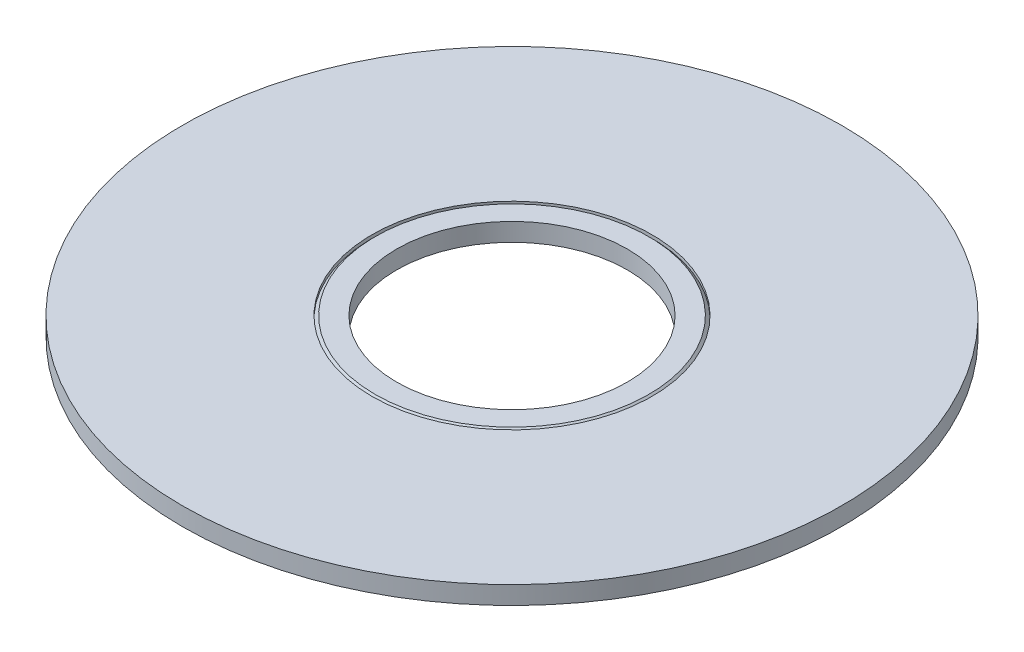
from build123d import *

# Parameters (mm, degrees)
SKETCH1_R           = 42.5
SKETCH1_R_2         = 35
BOSS_EXTRUDE1_DEPTH = 5.5
CHAMFER1_SIZE       = 1
BOSS_EXTRUDE2_START = -5.5
SKETCH2_R           = 100
SKETCH2_R_2         = 42.5
BOSS_EXTRUDE2_DEPTH = 5.5


with BuildPart() as part:
    # Sketch1 → Boss-Extrude1 (new body)
    with BuildSketch(Plane(origin=(0, 0, 0), x_dir=(1, 0, 0), z_dir=(0, 1, 0))):
        with Locations(Location((0, 0, 0), (0, 0, 270))):
            Circle(SKETCH1_R)
        with Locations(Location((0, 0, 0), (0, 0, 270))):
            Circle(SKETCH1_R_2, mode=Mode.SUBTRACT)
    extrude(amount=BOSS_EXTRUDE1_DEPTH)

    # Chamfer1
    chamfer1_edges = [part.edges().sort_by_distance(p)[0] for p in [
        (0, 0, -42.5),
        (0, 5.5, -42.5),
    ]]
    chamfer(chamfer1_edges, length=CHAMFER1_SIZE)

    # Sketch2 → Boss-Extrude2 (add)
    with BuildSketch(Plane(origin=(0, 5.5, 0), x_dir=(1, 0, 0), z_dir=(0, 1, 0)).offset(BOSS_EXTRUDE2_START)):
        with Locations(Location((0, 0, 0), (0, 0, 270))):
            Circle(SKETCH2_R)
        with Locations(Location((0, 0, 0), (0, 0, 270))):
            Circle(SKETCH2_R_2, mode=Mode.SUBTRACT)
    extrude(amount=BOSS_EXTRUDE2_DEPTH)


solid = part.part
